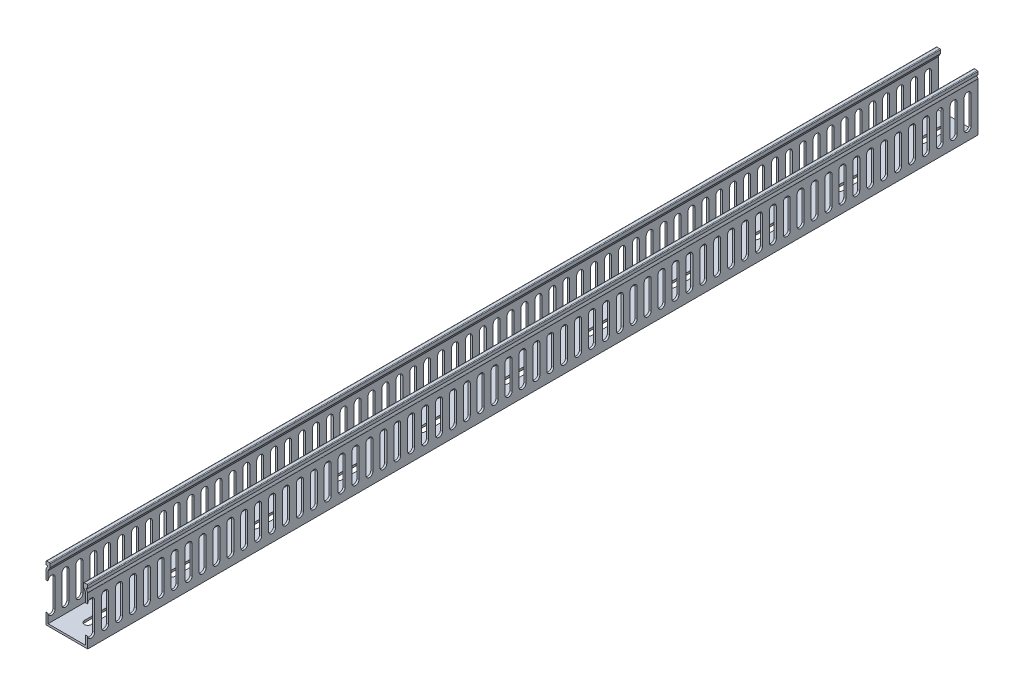
SolidWorks part; units mm, degrees
ref_plane "前基準面" through (0, 0, 0) normal (0, 0, 1) x (1, 0, 0)
ref_plane "上基準面" through (0, 0, 0) normal (0, 1, 0) x (1, 0, 0)
ref_plane "右基準面" through (0, 0, 0) normal (1, 0, 0) x (0, 0, -1)
sketch "草圖1" plane through (0, 0, 0) normal (0, 0, 1) x (1, 0, 0)
  line L0 (0, 0) -> (0, 65.5929) construction
  line L1 (14.9287, 35.1188) -> (13.9543, 36.7428)
  line L2 (14.3831, 37.5) -> (15, 37.5)
  line L3 (15, 37.5) -> (15, 39.5)
  line L4 (-15, 0) -> (15, 0)
  line L5 (15, 34.8615) -> (15, 0)
  line L6 (14.5, 40) -> (12.5, 40)
  line L7 (12, 39.5) -> (12, 37.223)
  line L8 (12.0713, 36.9658) -> (13.4287, 34.7033)
  line L9 (13.5, 34.446) -> (13.5, 1.5)
  line L10 (13.5, 1.5) -> (-13.5, 1.5)
  line L11 (-13.5, 34.446) -> (-13.5, 1.5)
  line L12 (-12.0713, 36.9658) -> (-13.4287, 34.7033)
  line L13 (-12, 39.5) -> (-12, 37.223)
  line L14 (-14.5, 40) -> (-12.5, 40)
  line L15 (-15, 34.8615) -> (-15, 0)
  line L16 (-15, 37.5) -> (-15, 39.5)
  line L17 (-14.3831, 37.5) -> (-15, 37.5)
  line L18 (-14.9287, 35.1188) -> (-13.9543, 36.7428)
  arc A0 (13.9543, 36.7428) -> (14.3831, 37.5) centre (14.3831, 37) cw
  arc A1 (14.5, 40) -> (15, 39.5) centre (14.5, 39.5) cw
  arc A2 (12, 39.5) -> (12.5, 40) centre (12.5, 39.5) cw
  arc A3 (12.0713, 36.9658) -> (12, 37.223) centre (12.5, 37.223) cw
  arc A4 (13.5, 34.446) -> (13.4287, 34.7033) centre (13, 34.446) ccw
  arc A5 (15, 34.8615) -> (14.9287, 35.1188) centre (14.5, 34.8615) ccw
  arc A6 (-15, 34.8615) -> (-14.9287, 35.1188) centre (-14.5, 34.8615) cw
  arc A7 (-13.5, 34.446) -> (-13.4287, 34.7033) centre (-13, 34.446) cw
  arc A8 (-12.0713, 36.9658) -> (-12, 37.223) centre (-12.5, 37.223) ccw
  arc A9 (-12, 39.5) -> (-12.5, 40) centre (-12.5, 39.5) ccw
  arc A10 (-14.5, 40) -> (-15, 39.5) centre (-14.5, 39.5) ccw
  arc A11 (-13.9543, 36.7428) -> (-14.3831, 37.5) centre (-14.3831, 37) ccw
  point P15 (13.5, 37.5)
  point P18 (15, 40)
  point P27 (15, 35)
  point P47 (0, 1.5)
  point P49 (-15, 35)
  point P50 (-15, 40)
  point P51 (-13.5, 37.5)
  dimension "D2" = 1.5
  dimension "D3" = 1.5
  dimension "D10" = 0.5
  dimension "D4" = 35
  dimension "D5" = 1.5
  dimension "D1" = 15
  dimension "D6" = 3
  dimension "D7" = 2.5
  dimension "D8" = 2.5
  dimension "D9" = 1.5
extrude "伸長1" add sketch "草圖1" along normal blind 640
sketch "草圖2" plane through (-15, 0, 0) normal (-1, 0, 0) x (0, 0, 1)
  line L0 (0, 34.8615) -> (0, 0) construction
  line L2 (5, 28) -> (5, 8)
  line L4 (10, 28) -> (10, 8)
  arc A0 (10, 28) -> (5, 28) centre (7.5, 28) ccw
  arc A1 (5, 8) -> (10, 8) centre (7.5, 8) ccw
  dimension "D1" = 5
  dimension "D2" = 20
  dimension "D3" = 5
extrude "伸長2" cut sketch "草圖2" against normal through all
pattern_linear "直線複製排列1" count 130 spacing 10 along (0, 0, 1) of "伸長2"
sketch "草圖3" plane through (0, 0, 0) normal (0, -1, 0) x (1, 0, 0)
  line L2 (-2.5, 25) -> (-2.5, 10)
  line L4 (2.5, 25) -> (2.5, 10)
  arc A0 (2.5, 25) -> (-2.5, 25) centre (0, 25) ccw
  arc A1 (-2.5, 10) -> (2.5, 10) centre (0, 10) ccw
  dimension "D2" = 5
  dimension "D1" = 15
  dimension "D4" = 2.5
extrude "伸長3" cut sketch "草圖3" against normal through all
pattern_linear "直線複製排列2" count 25 spacing 60 along (0, 0, 1) of "伸長3"
